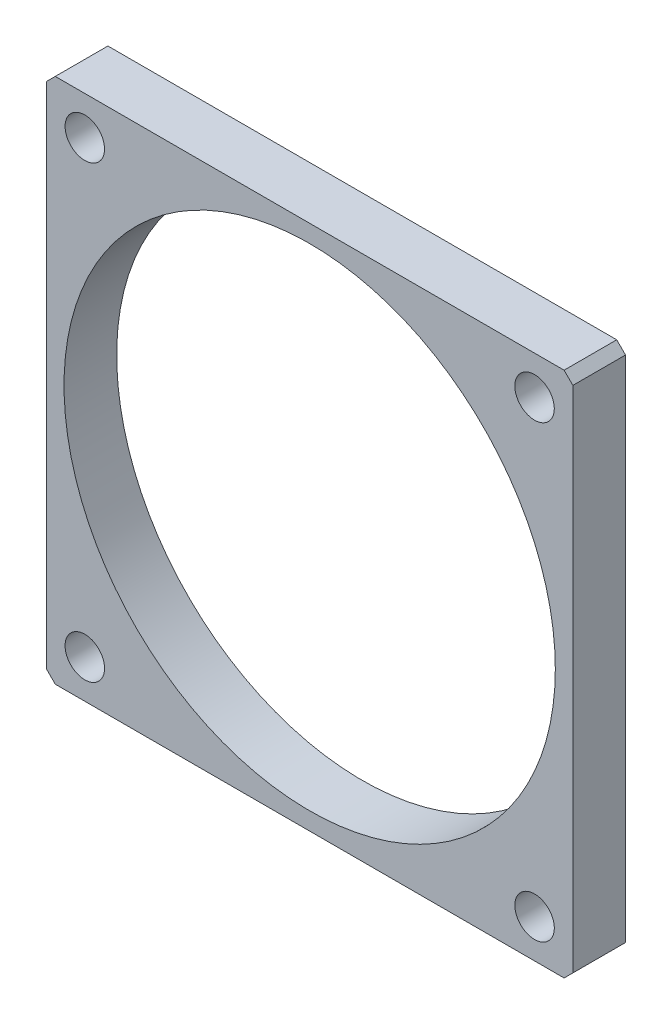
SolidWorks part; units mm, degrees
ref_plane "Front Plane" through (0, 0, 0) normal (0, 0, 1) x (1, 0, 0)
ref_plane "Top Plane" through (0, 0, 0) normal (0, 1, 0) x (1, 0, 0)
ref_plane "Right Plane" through (0, 0, 0) normal (1, 0, 0) x (0, 0, -1)
sketch "Sketch1" plane through (0, 0, 0) normal (0, 0, 1) x (1, 0, 0)
  line L1 (-60, 60) -> (60, 60)
  line L2 (-60, 60) -> (-60, -60)
  line L3 (-60, -60) -> (60, -60)
  line L4 (60, 60) -> (60, -60)
  line L5 (-60, 60) -> (60, -60) construction
  line L6 (-60, -60) -> (60, 60) construction
  point P0 (0, 0)
  dimension "D1" = 120
  dimension "D2" = 120
extrude "Boss-Extrude1" add sketch "Sketch1" along normal blind 12
sketch "Sketch2" plane through (0, 0, 12) normal (0, 0, 1) x (1, 0, 0)
  circle A0 centre (0, 0) radius 56
  dimension "D1" = 112
extrude "Cut-Extrude1" cut sketch "Sketch2" against normal through all
hole_wizard "M8 Clearance Hole1" positions "Sketch4" profile "Sketch3" hole size "M8" standard "ISO"
sketch "Sketch4" plane through (0, 0, 12) normal (0, 0, 1) x (1, 0, 0)
  line L0 (-60, 60) -> (0, 0) construction
  point P0 (-51.2652, 51.2652)
  dimension "D1" = 72.5
sketch "Sketch3" plane through (-51.2652, 51.2652, 12) normal (1, 0, 0) x (0, -1, 0)
  line L0 (0, 0) -> (0, 52.7039)
  line L1 (0, 52.7039) -> (4.5, 50)
  line L2 (4.5, 50) -> (4.5, 0)
  line L5 (4.5, 0) -> (0, 0)
  line L10 (0, 52.7039) -> (-4.5, 50) construction
  line L11 (0, -6.35) -> (0, 107.95) construction
  dimension "孔直径" = 9
  dimension "孔深度" = 50
  dimension "导头角度" = 118
pattern_circular "CirPattern1" count 4 over 360 about axis through (0, 0, 0) along (0, 0, 1) of "M8 Clearance Hole1"
chamfer "Chamfer1" distance 2 angle 45 4 edges at (60, 60, 6) (60, -60, 6) (-60, -60, 6) (-60, 60, 6)
